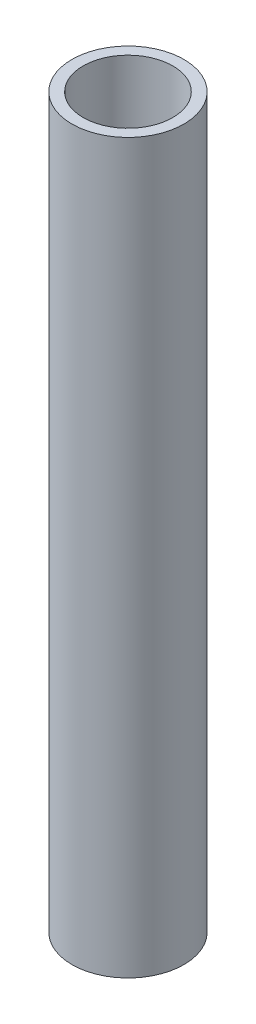
from build123d import *

# Parameters (mm, degrees)
SKETCH1_R           = 10
SKETCH1_R_2         = 8
BOSS_EXTRUDE1_DEPTH = 130


with BuildPart() as part:
    # Sketch1 → Boss-Extrude1 (new body)
    with BuildSketch(Plane(origin=(0, 0, 0), x_dir=(1, 0, 0), z_dir=(0, 1, 0))):
        with Locations(Location((0, 0, 0), (0, 0, 270))):
            Circle(SKETCH1_R)
        with Locations(Location((0, 0, 0), (0, 0, 270))):
            Circle(SKETCH1_R_2, mode=Mode.SUBTRACT)
    extrude(amount=BOSS_EXTRUDE1_DEPTH)


solid = part.part
